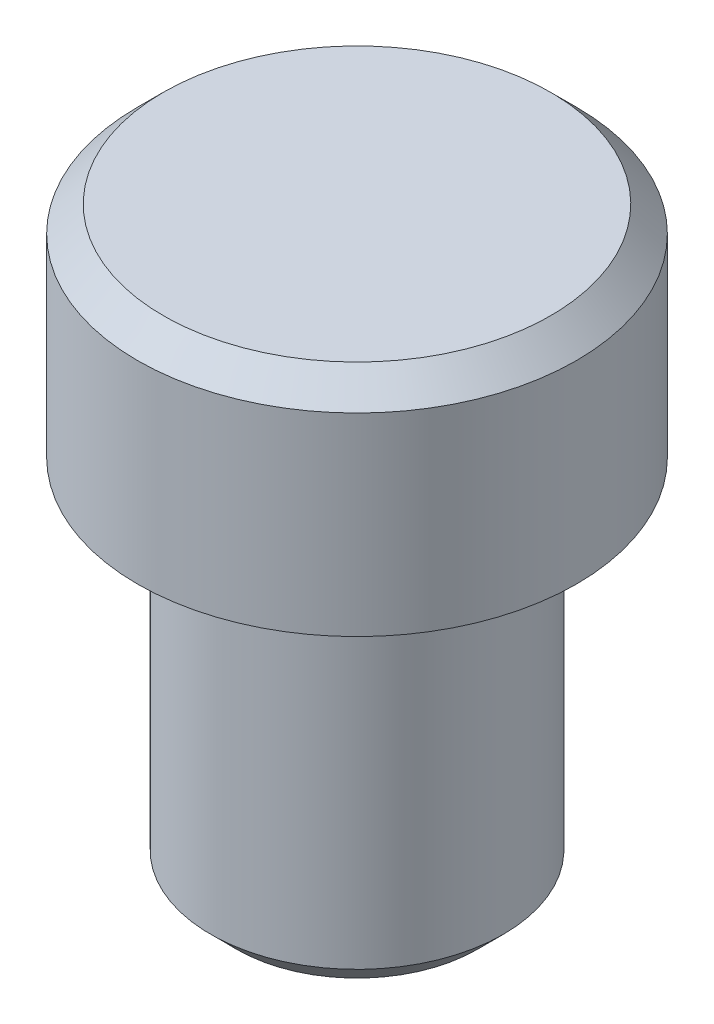
from build123d import *


with BuildPart() as part:
    # Sketch1 → Boss-Revolve (revolve)
    with BuildSketch(Plane.XY, mode=Mode.PRIVATE) as boss_revolve_sk:
        with BuildLine():
            Line((0, 0), (5.292893219, 0))
            Line((5.292893219, 0), (6, -0.707106781))
            Line((6, -0.707106781), (6, -6))
            Line((6, -6), (5, -6))
            Line((5, -6), (4.5, -5.5))
            Line((4.5, -5.5), (4, -5.5))
            ThreePointArc((4, -5.5), (3.646446609, -5.646446609), (3.5, -6))
            Line((3.5, -6), (3.5, -6.5))
            Line((3.5, -6.5), (4, -7))
            Line((4, -7), (4, -15.292893219))
            Line((4, -15.292893219), (3.292893219, -16))
            Line((3.292893219, -16), (0, -16))
            Line((0, -16), (0, 0))
        make_face()
    revolve(boss_revolve_sk.sketch.rotate(Axis((0, 42.170539173, 0), (0, -1, 0)), 180), axis=Axis((0, 42.170539173, 0), (0, -1, 0)))


solid = part.part
